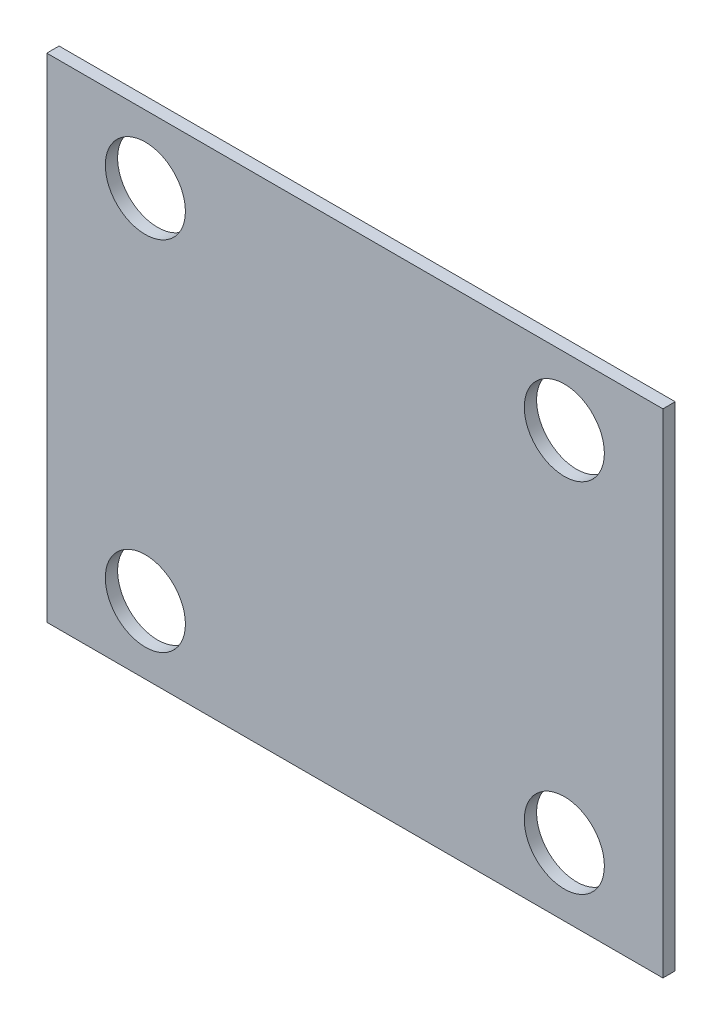
SolidWorks part; units mm, degrees
material "PF"
ref_plane "前视基准面" through (0, 0, 0) normal (0, 0, 1) x (1, 0, 0)
ref_plane "上视基准面" through (0, 0, 0) normal (0, 1, 0) x (1, 0, 0)
ref_plane "右视基准面" through (0, 0, 0) normal (1, 0, 0) x (0, 0, -1)
sketch "草图1" plane through (0, 0, 0) normal (0, 0, 1) x (1, 0, 0)
  line L1 (-50, 40) -> (50, 40)
  line L2 (-50, 40) -> (-50, -40)
  line L3 (-50, -40) -> (50, -40)
  line L4 (50, 40) -> (50, -40)
  line L5 (0, -40) -> (0, 40) construction
  line L6 (-50, 0) -> (50, 0) construction
  point P0 (0, 0)
  dimension "D1" = 100
  dimension "D2" = 80
extrude "凸台-拉伸1" add sketch "草图1" along normal blind 2
sketch "草图2" plane through (0, 0, 2) normal (0, 0, 1) x (1, 0, 0)
  line L1 (-34, 29) -> (34, 29) construction
  line L2 (-34, 29) -> (-34, -29) construction
  line L3 (-34, -29) -> (34, -29) construction
  line L4 (34, 29) -> (34, -29) construction
  line L5 (0, -29) -> (0, 29) construction
  line L6 (-34, 0) -> (34, 0) construction
  circle A0 centre (-34, 29) radius 6.5
  circle A1 centre (34, 29) radius 6.5
  circle A2 centre (34, -29) radius 6.5
  circle A3 centre (-34, -29) radius 6.5
  point P0 (0, 0)
  dimension "D3" = 13
  dimension "D1" = 68
  dimension "D2" = 58
extrude "切除-拉伸1" cut sketch "草图2" against normal blind 2
